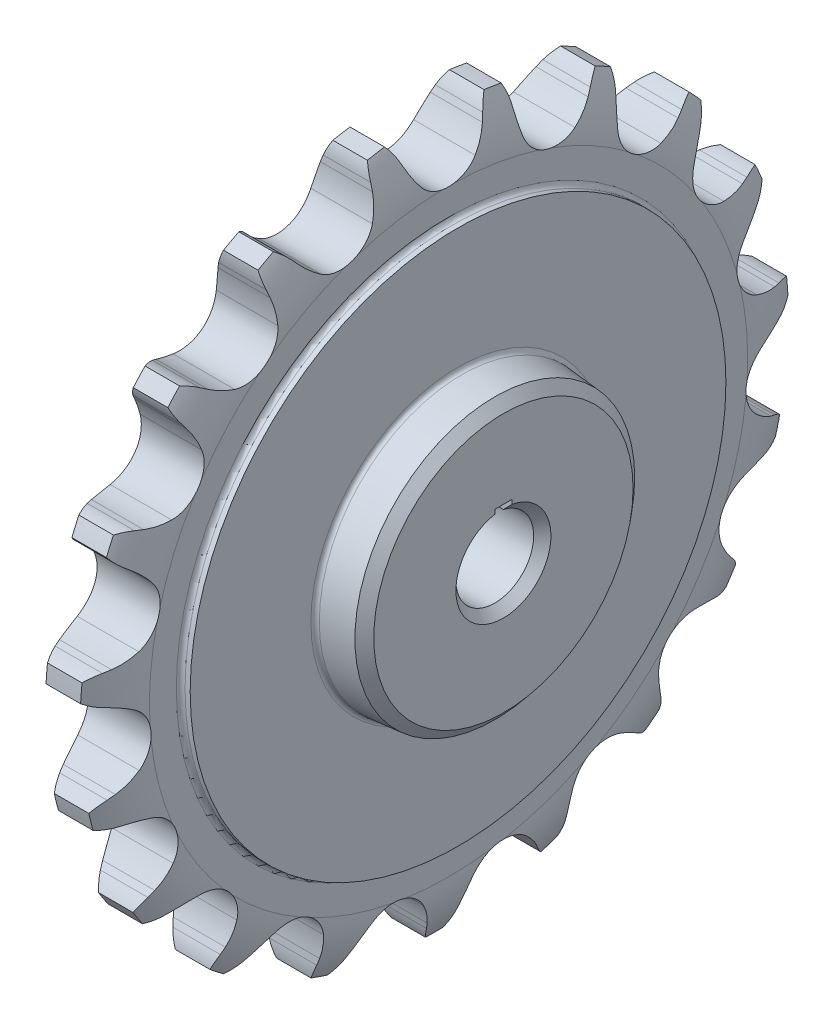
from build123d import *
from OCP.BRepFilletAPI import BRepFilletAPI_MakeChamfer

# Parameters (mm, degrees)
CUT_EXTRUDE1_DEPTH = 4.75
CIRPATTERN1_COUNT  = 19
SKETCH4_W          = 2
SKETCH4_H          = 1.512517806
CUT_EXTRUDE2_DEPTH = 60.782131128
FILLET1_R          = 0.508
CHAMFER1_SIZE      = 1
CHAMFER1_SIZE2     = 1.100062868


with BuildPart() as part:
    # Sketch1 → Revolve1 (revolve)
    with BuildSketch(Plane.XY, mode=Mode.PRIVATE) as revolve1_sk:
        with BuildLine():
            Line((-4.75, 4.5), (-4.75, 31))
            Line((-4.75, 31), (-4.15825, 31))
            ThreePointArc((-4.15825, 31), (-3.799039755, 31.148789755), (-3.65025, 31.508))
            Line((-3.65025, 31.508), (-3.65025, 34.619639763))
            ThreePointArc((-3.65025, 34.619639763), (-3.245836945, 37.918781526), (-1.99925, 41))
            Line((-1.99925, 41), (1.99925, 41))
            ThreePointArc((1.99925, 41), (3.245836945, 37.918781526), (3.65025, 34.619639763))
            Line((3.65025, 34.619639763), (3.65025, 31.508))
            ThreePointArc((3.65025, 31.508), (3.799039755, 31.148789755), (4.15825, 31))
            Line((4.15825, 31), (4.75, 31))
            Line((4.75, 31), (4.75, 4.5))
            Line((4.75, 4.5), (-4.75, 4.5))
        make_face()
    revolve(revolve1_sk.sketch.rotate(Axis((-6.35, 0, 0), (1, 0, 0)), 90), axis=Axis((-6.35, 0, 0), (1, 0, 0)))

    # Sketch2 → Cut-Extrude1 (cut, symmetric)
    with BuildSketch(Plane(origin=(0, 0, 0), x_dir=(0, 0, -1), z_dir=(1, 0, 0))):
        with BuildLine():
            Line((4.552244709, 38.426451297), (4.858741585, 39.1448403))
            ThreePointArc((4.858741585, 39.1448403), (5.250930322, 39.90290393), (5.750855114, 40.594675334))
            ThreePointArc((5.750855114, 40.594675334), (0, 41), (-5.750855114, 40.594675334))
            ThreePointArc((-5.750855114, 40.594675334), (-5.250930322, 39.90290393), (-4.858741585, 39.1448403))
            Line((-4.858741585, 39.1448403), (-4.552244709, 38.426451297))
            ThreePointArc((-4.552244709, 38.426451297), (-3.937302758, 37.212676935), (-3.168676608, 36.089905522))
            ThreePointArc((-3.168676608, 36.089905522), (0, 34.549839763), (3.168676608, 36.089905522))
            ThreePointArc((3.168676608, 36.089905522), (3.937302758, 37.212676935), (4.552244709, 38.426451297))
        make_face()
    cut_extrude1 = extrude(amount=CUT_EXTRUDE1_DEPTH, both=True, mode=Mode.SUBTRACT)

    # CirPattern1: Cut-Extrude1 ×19 about axis
    cirpattern1_axis = Axis((0, 0, 0), (1, 0, 0))
    for i in range(1, CIRPATTERN1_COUNT):
        add(cut_extrude1.rotate(cirpattern1_axis, i * 360 / CIRPATTERN1_COUNT), mode=Mode.SUBTRACT)

    # Sketch5 → Revolve2 (revolve)
    with BuildSketch(Plane.XY, mode=Mode.PRIVATE) as revolve2_sk:
        Polygon((-10, 4.5), (10, 4.5), (10, 16.104926129), (4.75, 16.564241612), (-4.75, 16.564241612), (-10, 16.104926129), align=None)
    revolve(revolve2_sk.sketch.rotate(Axis((0, 0, 0), (-1, 0, 0)), 90), axis=Axis((0, 0, 0), (-1, 0, 0)))

    # Sketch4 → Cut-Extrude2 (cut, through all)
    with BuildSketch(Plane.ZY.offset(4.75)):
        with Locations((0, 5.143741097)):
            Rectangle(SKETCH4_W, SKETCH4_H)
    cut_extrude2 = extrude(amount=-CUT_EXTRUDE2_DEPTH, mode=Mode.SUBTRACT)

    # Mirror1: Cut-Extrude2 across plane
    add(cut_extrude2.mirror(Plane(origin=(0, 0, 0), x_dir=(0, 0, 1), z_dir=(1, 0, 0))), mode=Mode.SUBTRACT)

    # Fillet1
    fillet1_edges = [part.edges().sort_by_distance(p)[0] for p in [
        (-4.75, 0, 16.564241612),
        (4.75, 0, 16.564241612),
    ]]
    fillet(fillet1_edges, radius=FILLET1_R)

    # Chamfer1: one chamfer whose edges measure the first distance from different faces: ONE call of the kernel's chamfer builder (chamfer() names one face for all edges)
    chamfer1_edges_1 = [part.edges().sort_by_distance(p)[0] for p in [
        (-10, 0, 16.104926129),
    ]]
    chamfer1_side_1 = [part.faces().sort_by_distance(p)[0] for p in [
        (-10, 0, 15.64941003),
    ]]
    chamfer1_edges_2 = [part.edges().sort_by_distance(p)[0] for p in [
        (10, 0, 16.104926129),
    ]]
    chamfer1_side_2 = [part.faces().sort_by_distance(p)[0] for p in [
        (7.606862441, 0, 16.314298535),
    ]]
    chamfer1_edges_3 = [part.edges().sort_by_distance(p)[0] for p in [
        (10, -4.5, 0),
        (-10, -4.5, 0),
    ]]
    chamfer1 = BRepFilletAPI_MakeChamfer(part.part.solid().wrapped)
    for e in chamfer1_edges_1:
        chamfer1.Add(CHAMFER1_SIZE, CHAMFER1_SIZE2, e.wrapped, chamfer1_side_1[0].wrapped)  # the first distance lies on this face
    for e in chamfer1_edges_2:
        chamfer1.Add(CHAMFER1_SIZE, CHAMFER1_SIZE2, e.wrapped, chamfer1_side_2[0].wrapped)  # the first distance lies on this face
    for e in chamfer1_edges_3:
        chamfer1.Add(CHAMFER1_SIZE, e.wrapped)
    add(Compound.cast(chamfer1.Shape()), mode=Mode.REPLACE)


solid = part.part
